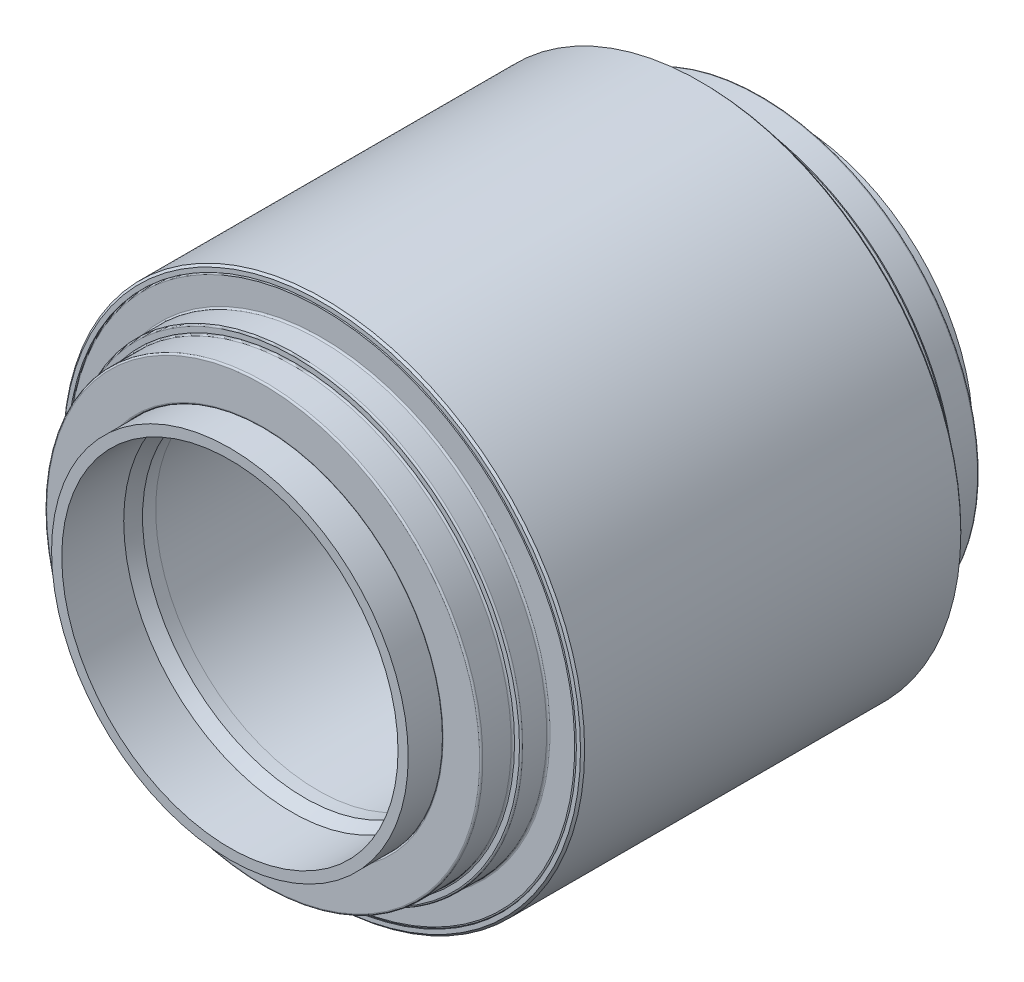
SolidWorks part; units mm, degrees
material "普通碳钢"
ref_plane "Front plane" through (0, 0, 0) normal (0, 0, 1) x (1, 0, 0)
ref_plane "Top plane" through (0, 0, 0) normal (0, 1, 0) x (1, 0, 0)
ref_plane "Right plane" through (0, 0, 0) normal (1, 0, 0) x (0, 0, -1)
sketch "Sketch1" plane through (0, 0, 0) normal (1, 0, 0) x (0, 0, -1)
  line L0 (-191.0635, 0) -> (0, 0) construction
  line L1 (0, 0) -> (0, 192.8904) construction
  line L2 (92.075, 126.2063) -> (-92.075, 126.2063)
  line L3 (-92.075, 126.2063) -> (-92.075, 109.625)
  line L4 (-78.915, 123.2063) -> (-78.915, 121.7063)
  line L5 (100.382, 78.5749) -> (-100.382, 78.5749)
  line L6 (-71.1849, 97.6694) -> (-66.9871, 119.2652)
  line L7 (-92.075, 123.2063) -> (-78.915, 123.2063)
  line L8 (-78.915, 121.7063) -> (-18, 109.24)
  line L9 (-15, 78.5749) -> (-15, 86.5749)
  line L10 (-15, 83.5749) -> (15, 83.5749)
  line L11 (-15, 86.5749) -> (-22.4056, 86.5749)
  line L12 (-136.652, 81.42) -> (-136.652, 86.36)
  line L13 (-22.0093, 88.6137) -> (-71.1849, 97.6694)
  line L14 (-136.652, 81.42) -> (-106.652, 81.42)
  line L15 (-71.9808, 93.5749) -> (-94.032, 93.5749)
  line L16 (-104.032, 86.36) -> (-94.032, 85.4851)
  line L17 (-22.0093, 88.6137) -> (-18, 109.24)
  line L18 (-18, 109.24) -> (18, 109.24)
  line L19 (-20.0047, 98.9269) -> (-69.086, 108.4673) construction
  line L20 (-136.652, 86.36) -> (-104.032, 86.36)
  line L21 (-78.915, 121.7063) -> (-90.575, 121.7063)
  line L22 (-106.652, 81.42) -> (-100.382, 78.5749)
  line L23 (-94.032, 78.5749) -> (-94.032, 93.5749)
  line L24 (-92.075, 109.625) -> (-105.235, 109.625)
  line L25 (-105.235, 109.625) -> (-105.235, 105.625)
  line L26 (-105.235, 105.625) -> (-120.545, 105.625)
  line L27 (-120.545, 105.625) -> (-120.545, 86.36)
  line L28 (90.575, 108.125) -> (90.575, 121.7063)
  line L29 (-119.045, 86.36) -> (-119.045, 104.125)
  line L30 (-119.045, 104.125) -> (-103.735, 104.125)
  line L31 (-103.735, 86.36) -> (-103.735, 108.125)
  line L32 (-103.735, 108.125) -> (-90.575, 108.125)
  line L33 (-90.575, 108.125) -> (-90.575, 121.7063)
  line L34 (103.735, 108.125) -> (90.575, 108.125)
  line L35 (103.735, 86.36) -> (103.735, 108.125)
  line L36 (119.045, 104.125) -> (93.416, 104.125)
  line L37 (119.045, 86.36) -> (119.045, 104.125)
  line L38 (120.545, 105.625) -> (120.545, 86.36)
  line L39 (105.235, 105.625) -> (120.545, 105.625)
  line L40 (105.235, 109.625) -> (105.235, 105.625)
  line L41 (92.075, 109.625) -> (105.235, 109.625)
  line L42 (94.032, 78.5749) -> (94.032, 93.5749)
  line L43 (106.652, 81.42) -> (100.382, 78.5749)
  line L44 (78.915, 121.7063) -> (90.575, 121.7063)
  line L45 (136.652, 86.36) -> (104.032, 86.36)
  line L46 (22.0093, 88.6137) -> (18, 109.24)
  line L47 (104.032, 86.36) -> (94.032, 85.4851)
  line L48 (71.9808, 93.5749) -> (94.032, 93.5749)
  line L49 (136.652, 81.42) -> (106.652, 81.42)
  line L50 (22.0093, 88.6137) -> (71.1849, 97.6694)
  line L51 (136.652, 81.42) -> (136.652, 86.36)
  line L52 (15, 86.5749) -> (22.4056, 86.5749)
  line L53 (15, 78.5749) -> (15, 86.5749)
  line L54 (78.915, 121.7063) -> (18, 109.24)
  line L55 (92.075, 123.2063) -> (78.915, 123.2063)
  line L56 (71.1849, 97.6694) -> (66.9871, 119.2652)
  line L57 (78.915, 123.2063) -> (78.915, 121.7063)
  line L58 (92.075, 126.2063) -> (92.075, 109.625)
  point P63 (0, 109.24)
  point P71 (0, 83.5749)
  point P75 (0, 78.5749)
  point P76 (0, 126.2063)
  dimension "D1" = 252.4125
  dimension "D2" = 184.15
  dimension "D3" = 3
  dimension "D4" = 11
  dimension "D5" = 1.5
  dimension "D6" = 1.5
  dimension "D7" = 22
  dimension "D8" = 157.1498
  dimension "D9" = 15
  dimension "D10" = 5
  dimension "D11" = 5
  dimension "D12" = 50
  dimension "D13" = 15
  dimension "D14" = 218.48
  dimension "D15" = 18
  dimension "D16" = 136.652
  dimension "D17" = 10
  dimension "D18" = 3
  dimension "D19" = 172.72
  dimension "D20" = 162.84
  dimension "D21" = 42.62
  dimension "D22" = 6.35
  dimension "D23" = 219.25
  dimension "D24" = 41.63
  dimension "D25" = 1.5
  dimension "D26" = 1.5
  dimension "D27" = 1.5
  dimension "D28" = 1.5
  dimension "D29" = 13.16
  dimension "D30" = 13.16
  dimension "D31" = 4
  dimension "D32" = 30
ref_plane "Plane1" through (0, 0, 0) normal (0.9927, -0.1205, 0) x (0, 0, -1)
sketch "Sketch2" plane through (0, 0, 0) normal (1, 0, 0) x (0, 0, -1)
  line L0 (15, 78.5749) -> (15, 86.5749) construction
  line L1 (100.382, 78.5749) -> (-100.382, 78.5749) construction
  line L2 (-15, 78.5749) -> (-15, 86.5749) construction
  line L3 (-15, 83.5749) -> (15, 83.5749) construction
  line L4 (15, 78.5749) -> (15, 83.5749)
  line L5 (15, 78.5749) -> (-15, 78.5749)
  line L6 (-15, 78.5749) -> (-15, 83.5749)
  line L7 (-15, 83.5749) -> (15, 83.5749)
  line L8 (-191.0635, 0) -> (0, 0) construction
revolve "Revolve1" add sketch "Sketch2" angle 360 about L8
sketch "Sketch3" plane through (0, 0, 0) normal (1, 0, 0) x (0, 0, -1)
  line L0 (-22.0093, 88.6137) -> (-71.1849, 97.6694) construction
  line L1 (-71.1849, 97.6694) -> (-66.9871, 119.2652) construction
  line L2 (-71.9808, 93.5749) -> (-94.032, 93.5749) construction
  line L3 (-94.032, 78.5749) -> (-94.032, 93.5749) construction
  line L4 (100.382, 78.5749) -> (-100.382, 78.5749) construction
  line L5 (-15, 78.5749) -> (-15, 86.5749) construction
  line L6 (-15, 86.5749) -> (-22.4056, 86.5749) construction
  line L7 (-22.0093, 88.6137) -> (-18, 109.24) construction
  line L8 (-22.0093, 88.6137) -> (-71.1849, 97.6694)
  line L9 (-71.1849, 97.6694) -> (-71.9808, 93.5749)
  line L10 (-71.9808, 93.5749) -> (-94.032, 93.5749)
  line L11 (-94.032, 78.5749) -> (-94.032, 93.5749)
  line L12 (-15, 78.5749) -> (-94.032, 78.5749)
  line L13 (-15, 78.5749) -> (-15, 86.5749)
  line L14 (-15, 86.5749) -> (-22.4056, 86.5749)
  line L15 (-22.0093, 88.6137) -> (-22.4056, 86.5749)
  line L16 (-191.0635, 0) -> (0, 0) construction
revolve "Revolve2" add sketch "Sketch3" angle 360 about L16
sketch "Sketch4" plane through (0, 0, 0) normal (1, 0, 0) x (0, 0, -1)
  line L0 (-94.032, 78.5749) -> (-94.032, 93.5749) construction
  line L1 (-136.652, 81.42) -> (-136.652, 86.36) construction
  line L2 (-136.652, 86.36) -> (-104.032, 86.36) construction
  line L3 (-104.032, 86.36) -> (-94.032, 85.4851) construction
  line L4 (-136.652, 81.42) -> (-106.652, 81.42) construction
  line L5 (-106.652, 81.42) -> (-100.382, 78.5749) construction
  line L6 (100.382, 78.5749) -> (-100.382, 78.5749) construction
  line L7 (-94.032, 78.5749) -> (-94.032, 85.4851)
  line L8 (-136.652, 81.42) -> (-136.652, 86.36)
  line L9 (-136.652, 86.36) -> (-104.032, 86.36)
  line L10 (-104.032, 86.36) -> (-94.032, 85.4851)
  line L11 (-136.652, 81.42) -> (-106.652, 81.42)
  line L12 (-106.652, 81.42) -> (-100.382, 78.5749)
  line L13 (-94.032, 78.5749) -> (-100.382, 78.5749)
  line L14 (-191.0635, 0) -> (0, 0) construction
revolve "Revolve3" add sketch "Sketch4" angle 360 about L14
sketch "Sketch5" plane through (0, 0, 0) normal (1, 0, 0) x (0, 0, -1)
  line L0 (-119.045, 86.36) -> (-119.045, 104.125) construction
  line L1 (-119.045, 104.125) -> (-103.735, 104.125) construction
  line L2 (-103.735, 86.36) -> (-103.735, 108.125) construction
  line L3 (-136.652, 86.36) -> (-104.032, 86.36) construction
  line L4 (-119.045, 86.36) -> (-119.045, 104.125)
  line L5 (-119.045, 104.125) -> (-103.735, 104.125)
  line L6 (-103.735, 86.36) -> (-103.735, 104.125)
  line L7 (-119.045, 86.36) -> (-103.735, 86.36)
  line L8 (-191.0635, 0) -> (0, 0) construction
revolve "Revolve4" add sketch "Sketch5" angle 360 about L8
sketch "Sketch6" plane through (0, 0, 0) normal (1, 0, 0) x (0, 0, -1)
  line L0 (-78.915, 123.2063) -> (-78.915, 121.7063) construction
  line L1 (-92.075, 126.2063) -> (-92.075, 109.625) construction
  line L2 (-78.915, 121.7063) -> (-90.575, 121.7063) construction
  line L3 (-92.075, 123.2063) -> (-78.915, 123.2063) construction
  line L4 (-90.575, 108.125) -> (-90.575, 121.7063) construction
  line L5 (-92.075, 109.625) -> (-105.235, 109.625) construction
  line L6 (-103.735, 108.125) -> (-90.575, 108.125) construction
  line L7 (-103.735, 86.36) -> (-103.735, 108.125) construction
  line L8 (-105.235, 109.625) -> (-105.235, 105.625) construction
  line L9 (-105.235, 105.625) -> (-120.545, 105.625) construction
  line L10 (-119.045, 104.125) -> (-103.735, 104.125) construction
  line L11 (-119.045, 86.36) -> (-119.045, 104.125) construction
  line L12 (-136.652, 86.36) -> (-104.032, 86.36) construction
  line L13 (-120.545, 105.625) -> (-120.545, 86.36) construction
  line L14 (-78.915, 123.2063) -> (-78.915, 121.7063)
  line L15 (-92.075, 123.2063) -> (-92.075, 109.625)
  line L16 (-78.915, 121.7063) -> (-90.575, 121.7063)
  line L17 (-92.075, 123.2063) -> (-78.915, 123.2063)
  line L18 (-90.575, 108.125) -> (-90.575, 121.7063)
  line L19 (-92.075, 109.625) -> (-105.235, 109.625)
  line L20 (-103.735, 108.125) -> (-90.575, 108.125)
  line L21 (-103.735, 104.125) -> (-103.735, 108.125)
  line L22 (-105.235, 109.625) -> (-105.235, 105.625)
  line L23 (-105.235, 105.625) -> (-120.545, 105.625)
  line L24 (-119.045, 104.125) -> (-103.735, 104.125)
  line L25 (-119.045, 86.36) -> (-119.045, 104.125)
  line L26 (-120.545, 86.36) -> (-119.045, 86.36)
  line L27 (-120.545, 105.625) -> (-120.545, 86.36)
  line L28 (-191.0635, 0) -> (0, 0) construction
revolve "Revolve5" add sketch "Sketch6" angle 360 about L28
sketch "Sketch7" plane through (0, 0, 0) normal (-0.9927, 0.1205, 0) x (0, 0, -1)
  line L0 (-20.0047, -98.2056) -> (-69.086, -107.6765) construction
  line L1 (-71.1849, -96.9573) -> (-66.9871, -118.3957) construction
  line L2 (-22.0093, -87.9676) -> (-18, -108.4435) construction
  line L3 (-22.0093, -87.9676) -> (-71.1849, -96.9573) construction
  line L8 (-69.086, -107.6765) -> (19.9076, -90.504) construction
  line L9 (-71.1849, -96.9573) -> (-22.0093, -87.9676)
  line L10 (-20.0047, -98.2056) -> (-22.0093, -87.9676)
  line L11 (-20.0047, -98.2056) -> (-69.086, -107.6765)
  line L12 (-69.086, -107.6765) -> (-71.1849, -96.9573)
revolve "Revolve7" add sketch "Sketch7" angle 360 about L8
sketch "Sketch9" plane through (0, 0, 0) normal (1, 0, 0) x (0, 0, -1)
  line L0 (-191.0635, 0) -> (0, 0) construction
  line L1 (71.1849, 97.6694) -> (66.9871, 119.2652) construction
  line L2 (71.9808, 93.5749) -> (94.032, 93.5749) construction
  line L3 (94.032, 78.5749) -> (94.032, 93.5749) construction
  line L4 (100.382, 78.5749) -> (-100.382, 78.5749) construction
  line L5 (15, 78.5749) -> (15, 86.5749) construction
  line L6 (15, 86.5749) -> (22.4056, 86.5749) construction
  line L7 (22.0093, 88.6137) -> (18, 109.24) construction
  line L8 (22.0093, 88.6137) -> (71.1849, 97.6694) construction
  line L9 (71.1849, 97.6694) -> (71.9808, 93.5749)
  line L10 (71.9808, 93.5749) -> (94.032, 93.5749)
  line L11 (94.032, 78.5749) -> (94.032, 93.5749)
  line L12 (94.032, 78.5749) -> (15, 78.5749)
  line L13 (15, 78.5749) -> (15, 86.5749)
  line L14 (15, 86.5749) -> (22.4056, 86.5749)
  line L15 (22.0093, 88.6137) -> (22.4056, 86.5749)
  line L16 (22.0093, 88.6137) -> (71.1849, 97.6694)
revolve "Revolve9" add sketch "Sketch9" angle 360 about L0
sketch "Sketch10" plane through (0, 0, 0) normal (1, 0, 0) x (0, 0, -1)
  line L0 (106.652, 81.42) -> (100.382, 78.5749) construction
  line L1 (100.382, 78.5749) -> (-100.382, 78.5749) construction
  line L2 (94.032, 78.5749) -> (94.032, 93.5749) construction
  line L3 (104.032, 86.36) -> (94.032, 85.4851) construction
  line L4 (136.652, 86.36) -> (104.032, 86.36) construction
  line L5 (136.652, 81.42) -> (136.652, 86.36) construction
  line L6 (136.652, 81.42) -> (106.652, 81.42) construction
  line L7 (106.652, 81.42) -> (100.382, 78.5749)
  line L8 (100.382, 78.5749) -> (94.032, 78.5749)
  line L9 (94.032, 78.5749) -> (94.032, 85.4851)
  line L10 (104.032, 86.36) -> (94.032, 85.4851)
  line L11 (136.652, 86.36) -> (104.032, 86.36)
  line L12 (136.652, 81.42) -> (136.652, 86.36)
  line L13 (136.652, 81.42) -> (106.652, 81.42)
  line L14 (-191.0635, 0) -> (0, 0) construction
revolve "Revolve10" add sketch "Sketch10" angle 360 about L14
sketch "Sketch11" plane through (0, 0, 0) normal (1, 0, 0) x (0, 0, -1)
  line L0 (119.045, 86.36) -> (119.045, 104.125) construction
  line L1 (136.652, 86.36) -> (104.032, 86.36) construction
  line L2 (119.045, 104.125) -> (93.416, 104.125) construction
  line L4 (119.045, 86.36) -> (119.045, 104.125)
  line L5 (119.045, 86.36) -> (104.032, 86.36)
  line L6 (119.045, 104.125) -> (104.032, 104.125)
  line L7 (104.032, 86.36) -> (104.032, 104.125)
  line L8 (-191.0635, 0) -> (0, 0) construction
revolve "Revolve11" add sketch "Sketch11" angle 360 about L8
sketch "Sketch12" plane through (0, 0, 0) normal (1, 0, 0) x (0, 0, -1)
  line L0 (136.652, 86.36) -> (104.032, 86.36) construction
  line L1 (120.545, 105.625) -> (120.545, 86.36) construction
  line L2 (119.045, 86.36) -> (119.045, 104.125) construction
  line L3 (119.045, 104.125) -> (93.416, 104.125) construction
  line L5 (105.235, 109.625) -> (105.235, 105.625) construction
  line L6 (105.235, 105.625) -> (120.545, 105.625) construction
  line L7 (92.075, 109.625) -> (105.235, 109.625) construction
  line L8 (103.735, 108.125) -> (90.575, 108.125) construction
  line L9 (92.075, 126.2063) -> (92.075, 109.625) construction
  line L10 (90.575, 108.125) -> (90.575, 121.7063) construction
  line L11 (78.915, 121.7063) -> (90.575, 121.7063) construction
  line L12 (78.915, 123.2063) -> (78.915, 121.7063) construction
  line L13 (92.075, 123.2063) -> (78.915, 123.2063) construction
  line L14 (120.545, 86.36) -> (119.045, 86.36)
  line L15 (120.545, 105.625) -> (120.545, 86.36)
  line L16 (119.045, 86.36) -> (119.045, 104.125)
  line L17 (119.045, 104.125) -> (103.735, 104.125)
  line L18 (103.735, 104.125) -> (103.735, 108.125)
  line L19 (105.235, 109.625) -> (105.235, 105.625)
  line L20 (105.235, 105.625) -> (120.545, 105.625)
  line L21 (92.075, 109.625) -> (105.235, 109.625)
  line L22 (103.735, 108.125) -> (90.575, 108.125)
  line L23 (92.075, 123.2063) -> (92.075, 109.625)
  line L24 (90.575, 108.125) -> (90.575, 121.7063)
  line L25 (78.915, 121.7063) -> (90.575, 121.7063)
  line L26 (78.915, 123.2063) -> (78.915, 121.7063)
  line L27 (92.075, 123.2063) -> (78.915, 123.2063)
  line L28 (0, 0) -> (-191.0635, 0) construction
revolve "Revolve12" add sketch "Sketch12" angle 360 about L28
sketch "Sketch13" plane through (0, 0, 0) normal (-0.9927, 0.1205, 0) x (0, 0, -1)
  line L3 (22.0093, -87.9676) -> (18, -108.4435) construction
  line L5 (18.0008, -108.4447) -> (20.0057, -98.2058)
  line L6 (20.0057, -98.2058) -> (69.1017, -107.6018)
  line L7 (66.9879, -118.3968) -> (69.1017, -107.6018)
  line L8 (71.1849, -96.9573) -> (66.9871, -118.3957) construction
  line L9 (20.0047, -98.2056) -> (69.1017, -107.6018) construction
  line L10 (66.9879, -118.3968) -> (18.0008, -108.4447)
  line L12 (78.915, -120.8189) -> (18, -108.4435) construction
  dimension "D2" = 0.001
  dimension "D3" = 0.001
  dimension "D4" = 11
  dimension "D5" = 0.001
revolve "Revolve13" add sketch "Sketch13" angle 360 about L6
sketch "Sketch8" plane through (0, 0, 0) normal (1, 0, 0) x (0, 0, -1)
  line L0 (-78.915, 123.2063) -> (-78.915, 121.7063) construction
  line L1 (78.915, 123.2063) -> (78.915, 121.7063) construction
  line L2 (92.075, 126.2063) -> (92.075, 109.625) construction
  line L3 (92.075, 123.2063) -> (78.915, 123.2063) construction
  line L4 (92.075, 126.2063) -> (-92.075, 126.2063) construction
  line L5 (-92.075, 123.2063) -> (-78.915, 123.2063) construction
  line L6 (-78.915, 121.7063) -> (-18, 109.24) construction
  line L7 (-18, 109.24) -> (18, 109.24) construction
  line L8 (78.915, 121.7063) -> (18, 109.24) construction
  line L9 (-78.915, 123.2063) -> (-78.915, 121.7063)
  line L10 (78.915, 123.2063) -> (78.915, 121.7063)
  line L11 (92.075, 126.2063) -> (92.075, 123.2063)
  line L12 (92.075, 123.2063) -> (78.915, 123.2063)
  line L13 (92.075, 126.2063) -> (-92.075, 126.2063)
  line L14 (-92.075, 123.2063) -> (-78.915, 123.2063)
  line L15 (-78.915, 121.7063) -> (-18, 109.24)
  line L16 (-18, 109.24) -> (18, 109.24)
  line L17 (78.915, 121.7063) -> (18, 109.24)
  line L18 (-92.075, 126.2063) -> (-92.075, 109.625) construction
  line L19 (-92.075, 126.2063) -> (-92.075, 123.2063)
  line L20 (-191.0635, 0) -> (0, 0) construction
revolve "Revolve8" add sketch "Sketch8" angle 360 about L20
fillet "Fillet1" radius 0.8 6 edges at (123.2063, 0, 92.075) (105.625, 0, 120.545) (86.36, 0, 120.545) (109.625, 0, 105.235) (105.625, 0, 105.235) (109.625, 0, 92.075)
fillet "Fillet2" radius 0.8 6 edges at (-109.625, 0, -92.075) (-123.2063, 0, -92.075) (-86.36, 0, -120.545) (-105.625, 0, -120.545) (-105.625, 0, -105.235) (-109.625, 0, -105.235)
chamfer "Chamfer1" distance 1 angle 45 2 edges at (126.2063, 0, -92.075) (126.2063, 0, 92.075)
pattern_circular "CirPattern5" count 26 over 360 about axis through (0, 0, 191.0635) along (0, 0, -1) of "Revolve7"
pattern_circular "CirPattern7" count 26 over 360 about axis through (0, 0, 191.0635) along (0, 0, -1) of "Revolve13"
sketch "Sketch15" plane through (0, 0, 0) normal (0, 1, 0) x (1, 0, 0)
  line L0 (0, 0) -> (0, 141.3183) construction
  line L1 (81.42, 136.652) -> (-81.42, 136.652) construction
  circle A0 centre (0, 136.652) radius 3
  dimension "D1" = 6
extrude "Cut-Extrude3" cut sketch "Sketch15" along normal through all
